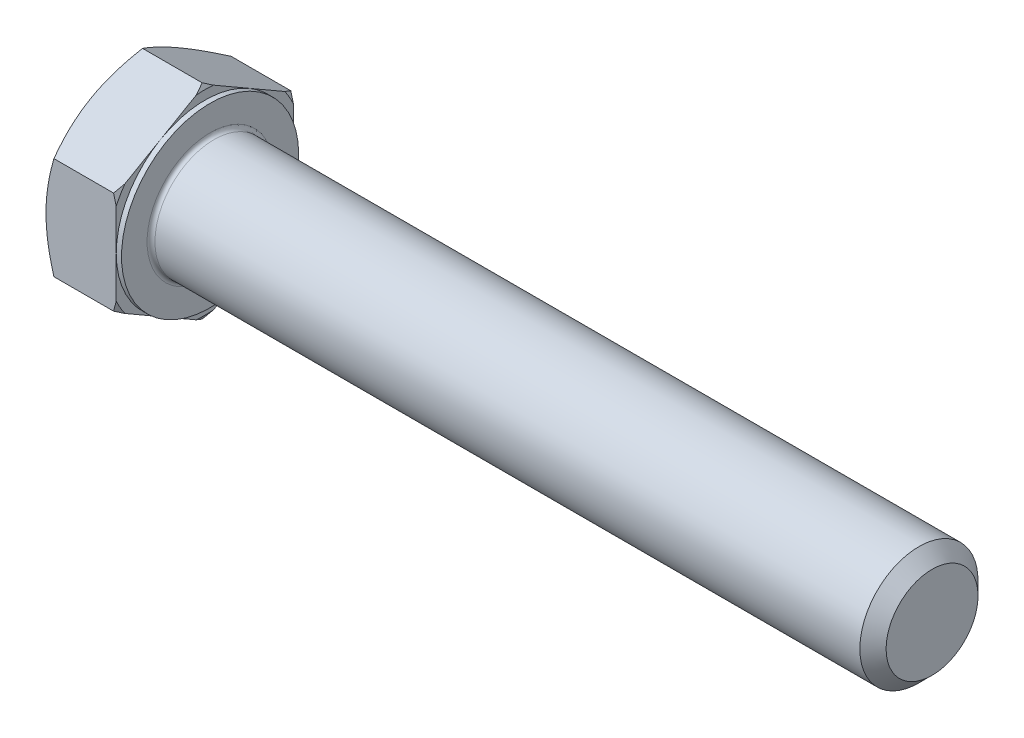
SolidWorks part; units mm, degrees
extrude "基体-拉伸" add sketch "草图1" along normal blind 11.5
sketch "草图1" plane through (0, 0, 0) normal (1, 0, 0) x (0, 0, -1)
  line L0 (13.5, 7.7942) -> (13.5, -7.7942)
  line L1 (-13.5, 7.7942) -> (-13.5, -7.7942)
  line L2 (13.5, -7.7942) -> (0, -15.5885)
  line L3 (0, -15.5885) -> (-13.5, -7.7942)
  line L4 (13.5, 7.7942) -> (0, 15.5885)
  line L5 (0, 15.5885) -> (-13.5, 7.7942)
revolve "切除-旋转1" cut sketch "草图3" angle 360 about L6
sketch "草图3" plane through (0, 0, 0) normal (0, 0, 1) x (1, 0, 0)
  line L0 (0, 13.5) -> (4.0925, 20.5885)
  line L1 (0, 15.5885) -> (0, 7.7942) construction
  line L2 (4.0925, 20.5885) -> (4.0925, 25.5885)
  line L3 (4.0925, 25.5885) -> (-10, 25.5885)
  line L4 (-10, 25.5885) -> (-10, 13.5)
  line L5 (-10, 13.5) -> (0, 13.5)
  line L6 (0, 0) -> (99.06, 0) construction
  line L7 (11.5, 15.5885) -> (0, 15.5885) construction
material "3.6级"
ref_plane "前视" through (0, 0, 0) normal (0, 0, 1) x (1, 0, 0)
ref_plane "上视" through (0, 0, 0) normal (0, 1, 0) x (1, 0, 0)
ref_plane "右视" through (0, 0, 0) normal (1, 0, 0) x (0, 0, -1)
sketch "草图2" plane through (0, 0, 0) normal (0, 0, 1) x (1, 0, 0)
  line L0 (0, 7.7942) -> (0, -7.7942) construction
  line L1 (0, 0) -> (121.5, 0)
  line L2 (0, 0) -> (0, 9)
  line L3 (0, 9) -> (27.8072, 9)
  line L4 (121.5, 0) -> (121.5, 6.835)
  line L5 (11.5, 15.5885) -> (11.5, 7.7942) construction
  line L7 (0, 0) -> (96.52, 0) construction
  line L8 (121.5, -6.835) -> (27.8072, -9) construction
  line L9 (0, -9) -> (27.8072, -9) construction
  line L10 (14, 15.24) -> (14, -1.27) construction
  line L11 (79.5, 15.24) -> (79.5, -1.27) construction
  line L12 (11.5, 7.7942) -> (11.5, -7.7942) construction
  line L13 (27.8072, 9) -> (121.5, 9)
  line L14 (121.5, 9) -> (121.5, 6.835)
revolve "凸台-旋转1" add sketch "草图2" angle 360 about L7
cosmetic thread "螺旋线1" parameters "Thread_length"=42, "Thread_minor"=13.67
sketch "草图5" plane through (0, 0, 0) normal (0, 0, 1) x (1, 0, 0)
  line L0 (11.5, 13.5) -> (7.4075, 20.5885)
  line L1 (11.5, 15.5885) -> (11.5, 7.7942) construction
  line L2 (7.4075, 20.5885) -> (7.4075, 25.5885)
  line L3 (7.4075, 25.5885) -> (17.4075, 25.5885)
  line L4 (17.4075, 25.5885) -> (17.4075, 13.5)
  line L5 (17.4075, 13.5) -> (11.5, 13.5)
  line L7 (11.5, 15.5885) -> (1.2058, 15.5885) construction
  line L8 (0, 0) -> (99.06, 0) construction
  line L9 (0, 0) -> (99.06, 0) construction
revolve "切除-旋转2" cut sketch "草图5" angle 360 about L8
sketch "草图4" plane through (0, 0, 0) normal (0, 0, 1) x (1, 0, 0)
  line L1 (11.5, 15.5885) -> (11.5, 7.7942) construction
  line L2 (11.5, 13.5) -> (10.7, 13.5)
  line L3 (11.5, 13.5) -> (11.5, 25.5885)
  line L4 (11.5, 25.5885) -> (10.7, 25.5885)
  line L5 (0, 0) -> (95.25, 0) construction
  line L6 (0, 0) -> (96.52, 0) construction
  line L7 (10.7, 13.5) -> (10.7, 25.5885)
  line L8 (10.2942, 15.5885) -> (1.2058, 15.5885) construction
revolve "切除-旋转3" cut sketch "草图4" angle 360 about L5
chamfer "倒角" distance 2 angle 45 1 edges at (121.5, 0, 9)
fillet "圆角" radius 0.6 1 edges at (11.5, 0, -9)
sketch "草图6" plane through (0, 0, 0) normal (0, 0, 1) x (1, 0, 0)
  line L0 (79.5, -6.835) -> (78.25, -9)
  line L1 (79.5, -6.835) -> (80.75, -9)
  line L2 (80.75, -9) -> (80.75, -11.25)
  line L3 (-3.175, 0) -> (5.1513, 0) construction
  line L5 (80.75, -11.25) -> (78.25, -11.25)
  line L6 (78.25, -11.25) -> (78.25, -9)
revolve "切除-旋转4" [suppressed] cut sketch "草图6" angle 360 about L3
pattern_linear "阵列(线性)1" [suppressed]
equation "\"D3@草图1\" = \"s@草图1\" / 2"
equation "\"D4@草图1\" = \"D3@草图1\""
equation "\"D5@草图1\" = \"D4@草图1\""
equation "\"Thread_minor@螺旋线1\" = \"Minor_dia@草图2\""
equation "\"D1@草图3\" = \"s@草图1\" / 2"
equation "\"D1@草图5\" = \"s@草图1\" / 2"
equation "\"Head_ch_ang@草图5\" = \"Head_ch_ang@草图3\""
equation "\"D1@草图4\" = \"s@草图1\""
equation "\"Thread_length@螺旋线1\" = ((sgn( (\"l@草图2\" - \"p@草图2\" ) - \"h@草图2\" )-1)*( (\"l@草图2\" - \"p@草图2\" ) - \"h@草图2\" ))/-2+ \"h@草图2\""
equation "\"Thread_minor@草图6\" = \"Minor_dia@草图2\""
equation "\"Diameter@草图6\" = \"m@草图2\""
equation "\"Overcut@草图6\" = \"m@草图2\" * 1.25"
equation "\"Start@草图6\" = \"k@基体-拉伸\" + \"l@草图2\" - \"Thread_length@螺旋线1\"  '---Non-countersunk---"
equation "\"Num_threads@阵列(线性)1\" = int( \"Thread_length@螺旋线1\" / \"p@草图2\" + 0.999 )  + 1"
equation "\"Advance@阵列(线性)1\" = \"Thread_length@螺旋线1\" /  (\"Num_threads@阵列(线性)1\" - 1) 'relax it"
equation "\"Num_threads@阵列(线性)1\" = \"Num_threads@阵列(线性)1\" - sgn( \"Num_threads@阵列(线性)1\" - 1) '---chamfered tips only---"
equation "\"Minor_dia@草图2\" = \"m@草图2\"-\"p@草图2\" * 1.732"
equation "\"D1@倒角\" = \"p@草图2\"*0.8"
